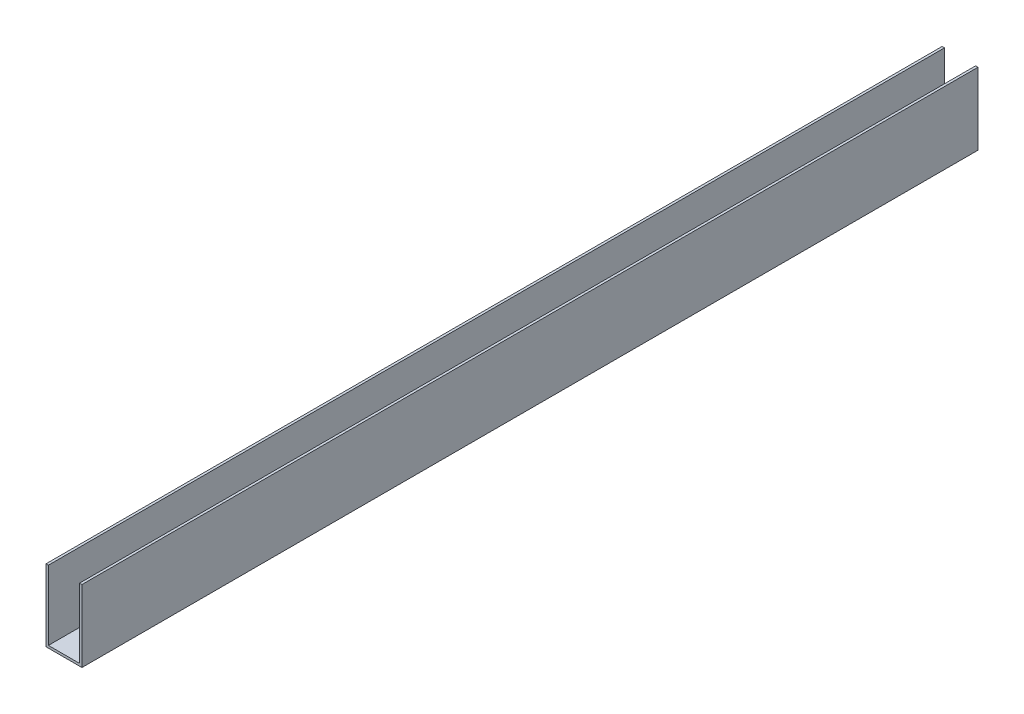
SolidWorks part; units mm, degrees
material "标准件"
ref_plane "前视基准面" through (0, 0, 0) normal (0, 0, 1) x (1, 0, 0)
ref_plane "上视基准面" through (0, 0, 0) normal (0, 1, 0) x (1, 0, 0)
ref_plane "右视基准面" through (0, 0, 0) normal (1, 0, 0) x (0, 0, -1)
sketch "草图1" plane through (0, 0, 0) normal (0, 0, 1) x (1, 0, 0)
  line L0 (0, 0) -> (0, 33.955) construction
  line L2 (-15, -30) -> (15, -30)
  line L3 (-15, -30) -> (-15, 30)
  line L4 (-15, 30) -> (15, 30)
  line L5 (15, -30) -> (15, 30)
  line L6 (-15, -30) -> (15, 30) construction
  line L7 (-15, 30) -> (15, -30) construction
  dimension "D1" = 30
  dimension "D2" = 60
extrude "凸台-拉伸1" add sketch "草图1" along normal mid plane 748
shell "抽壳1" thickness 2
